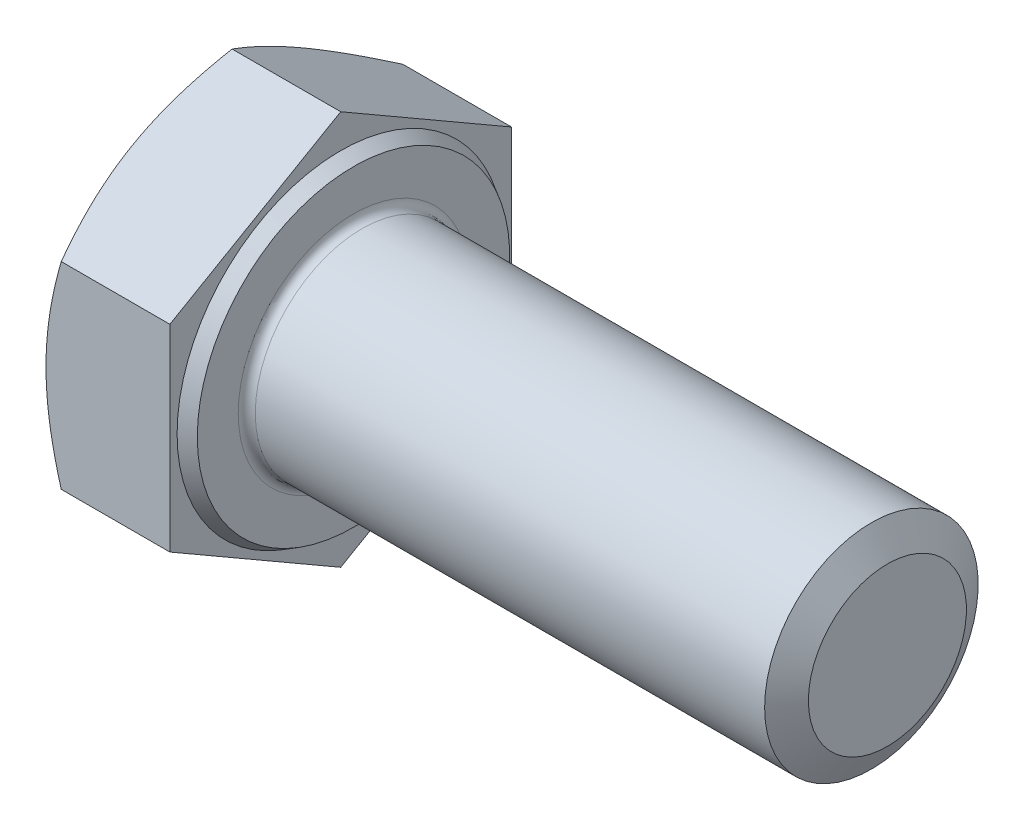
SolidWorks part; units mm, degrees
ref_plane "前视" through (0, 0, 0) normal (0, 0, 1) x (1, 0, 0)
ref_plane "上视" through (0, 0, 0) normal (0, 1, 0) x (1, 0, 0)
ref_plane "右视" through (0, 0, 0) normal (1, 0, 0) x (0, 0, -1)
sketch "草图1" plane through (0, 0, 0) normal (1, 0, 0) x (0, 0, -1)
  line L0 (8, 4.6188) -> (8, -4.6188)
  line L1 (-8, 4.6188) -> (-8, -4.6188)
  line L2 (8, -4.6188) -> (0, -9.2376)
  line L3 (0, -9.2376) -> (-8, -4.6188)
  line L4 (8, 4.6188) -> (0, 9.2376)
  line L5 (0, 9.2376) -> (-8, 4.6188)
  circle A0 centre (0, 0) radius 8.885 construction
  dimension "e" = 17.77
  dimension "s" = 16
  dimension "D2" = 120
  dimension "D3" = 8
  dimension "D4" = 8
  dimension "D5" = 8
extrude "基体-拉伸" add sketch "草图1" along normal blind 6.4
sketch "草图2" plane through (0, 0, 0) normal (0, 0, 1) x (1, 0, 0)
  line L0 (0, 4.6188) -> (0, -4.6188) construction
  line L1 (0, 0) -> (31.4, 0)
  line L2 (0, 0) -> (0, 5)
  line L3 (0, 5) -> (31.4, 5)
  line L4 (31.4, 0) -> (31.4, 3.701)
  line L5 (6.4, 9.2376) -> (6.4, 4.6188) construction
  line L6 (0, 0) -> (-11.2, 0) construction
  line L7 (0, 0) -> (15.7, 0) construction
  line L8 (31.4, -3.701) -> (90.335, -5) construction
  line L9 (0, -5) -> (90.335, -5) construction
  line L10 (7.9, 5) -> (7.9, 0) construction
  line L11 (6.4, 13.0554) -> (6.4, -1.27) construction
  line L12 (6.4, 4.6188) -> (6.4, -4.6188) construction
  line L14 (31.4, 5) -> (31.4, 3.701)
  dimension "l" = 25
  dimension "d" = 10
  dimension "Minor_dia" = 7.402
  dimension "p" = 1.5
  dimension "b" = 25
  dimension "da" = 11.2
revolve "凸台-旋转1" add sketch "草图2" angle 360 about L7
cosmetic thread "螺旋线1" parameters "Thread_length"=23.5, "Thread_minor"=7.402
sketch "草图3" plane through (0, 0, 0) normal (0, 0, 1) x (1, 0, 0)
  line L0 (0, 8) -> (3.6013, 14.2376)
  line L1 (0, 9.2376) -> (0, 4.6188) construction
  line L2 (3.6013, 14.2376) -> (3.6013, 19.2376)
  line L3 (3.6013, 19.2376) -> (-10, 19.2376)
  line L4 (-10, 19.2376) -> (-10, 8)
  line L5 (-10, 8) -> (0, 8)
  line L6 (0, 0) -> (99.06, 0) construction
  line L7 (6.4, 9.2376) -> (0, 9.2376) construction
  dimension "D1" = 8
  dimension "D2" = 5
  dimension "D3" = 10
  dimension "D4" = 5
  dimension "Head_ch_ang" = 30
revolve "切除-旋转1" cut sketch "草图3" angle 360 about L6
sketch "草图4" plane through (0, 0, 0) normal (0, 0, 1) x (1, 0, 0)
  line L0 (0, 0) -> (248.9073, 0) construction
  line L2 (6.4, 0) -> (6.4, 7.315) construction
  line L3 (6.4, -5) -> (6.4, 5) construction
  line L4 (6.4, 9.2376) -> (6.4, 4.6188) construction
  line L9 (6.4, 7.315) -> (5.8, 7.6614)
  line L10 (5.8, 7.6614) -> (5.8, 9.2376)
  line L11 (6.4, 9.2376) -> (0.7145, 9.2376) construction
  line L12 (5.8, 9.2376) -> (6.4, 9.2376)
  line L13 (6.4, 9.2376) -> (6.4, 7.315)
  dimension "D1" = 120
  dimension "c" = 0.6
  dimension "dw" = 14.63
revolve "切除-旋转3" cut sketch "草图4" angle 360 about L0
fillet "圆角" radius 0.4 1 edges at (6.4, 0, -5)
sketch "草图6" plane through (0, 0, 0) normal (0, 0, 1) x (1, 0, 0)
  line L0 (0, 0) -> (31.4, 0) construction
  line L1 (31.4, -5) -> (31.4, 5) construction
  line L2 (31.4, 0) -> (31.4, 5) construction
  line L4 (30.65, 5) -> (32.15, 5)
  line L5 (30.65, 5) -> (31.4, 3.701)
  line L6 (31.4, 3.701) -> (32.15, 5)
  dimension "D1" = 1.5
revolve "切除-旋转4" cut sketch "草图6" angle 360 about L0
pattern_linear "阵列(线性)1" [suppressed]
